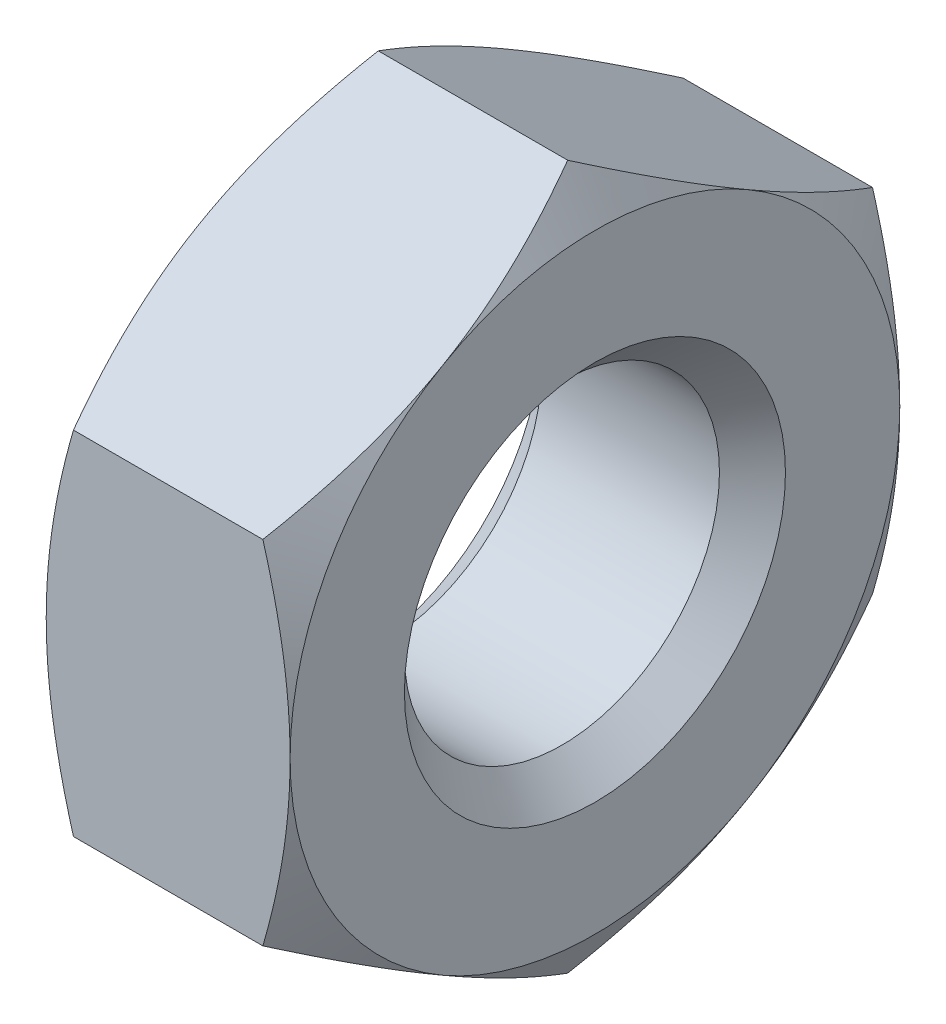
from build123d import *

# Parameters (mm, degrees)
BOSS_EXTRUDE1_DEPTH = 3.2


with BuildPart() as part:
    # Sketch1 → Boss-Extrude1 (new body)
    with BuildSketch(Plane(origin=(0, 0, 0), x_dir=(0, 0, -1), z_dir=(1, 0, 0))):
        Polygon((-4, 2.309401077), (-4, -2.309401077), (0, -4.618802154), (4, -2.309401077), (4, 2.309401077), (0, 4.618802154), align=None)
    extrude(amount=BOSS_EXTRUDE1_DEPTH)

    # Sketch2 → Cut-Revolve1 (revolve, cut)
    with BuildSketch(Plane.XY):
        Polygon((0, 4), (1.6, 6.771281292), (3.2, 4), (3.2, 10.2), (0, 10.2), align=None)
    revolve(axis=Axis((50, 0, 0), (-1, 0, 0)), mode=Mode.SUBTRACT)

    # Sketch3 → Cut-Revolve2 (revolve, cut)
    with BuildSketch(Plane.XY, mode=Mode.PRIVATE) as cut_revolve2_sk:
        Polygon((0, 0), (0, 2.5), (0.433, 2.067), (2.767, 2.067), (3.2, 2.5), (3.2, 0), align=None)
    revolve(cut_revolve2_sk.sketch.rotate(Axis((3.2, 0, 0), (-1, 0, 0)), 90), axis=Axis((3.2, 0, 0), (-1, 0, 0)), mode=Mode.SUBTRACT)


solid = part.part
